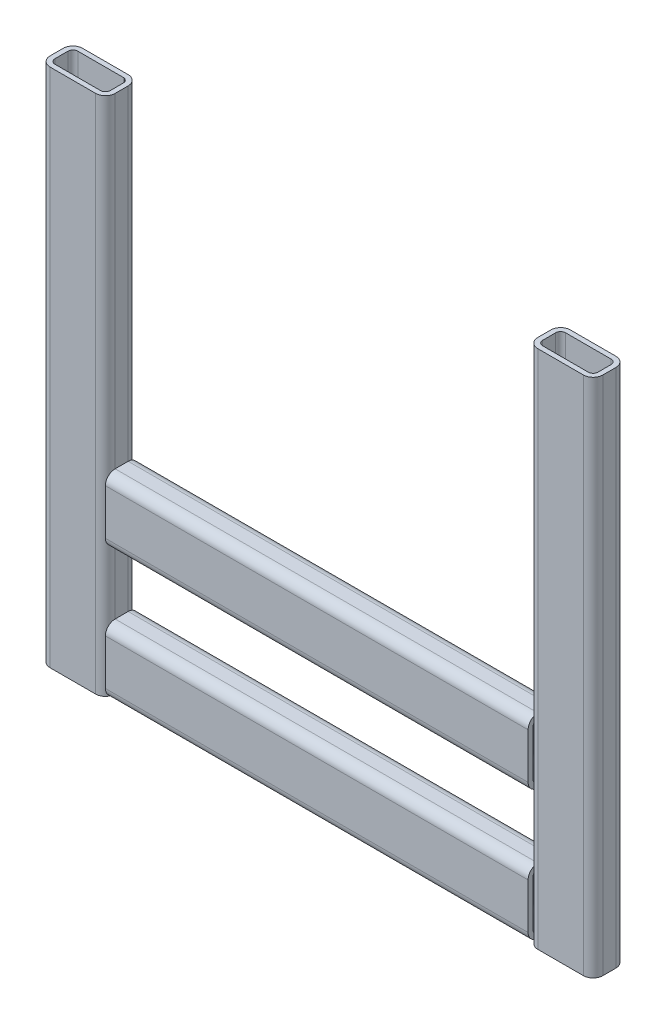
SolidWorks part; units mm, degrees
material "普通碳钢"
ref_plane "前视基准面" through (0, 0, 0) normal (0, 0, 1) x (1, 0, 0)
ref_plane "上视基准面" through (0, 0, 0) normal (0, 1, 0) x (1, 0, 0)
ref_plane "右视基准面" through (0, 0, 0) normal (1, 0, 0) x (0, 0, -1)
sketch3d "3D草图1"
  line L0 (0, 0, 0) -> (300, 0, 0)
  line L1 (300, 0, 0) -> (300, 300, 0)
  line L2 (0, 0, 0) -> (0, 300, 0)
  line L3 (0, 80, 0) -> (300, 80, 0)
  dimension "D1" = 300
  dimension "D2" = 300
  dimension "D3" = 80
other "矩形管 40 X 20 X 3(1)"
ref_plane "基准面1" through (0, 0, 0) normal (0, 1, 0) x (0, 0, -1)
sketch "Sketch1" plane through (0, 0, 0) normal (0, 1, 0) x (0, 0, -1)
  line L0 (-4, -17) -> (4, -17)
  line L1 (-7, -14) -> (-7, 14)
  line L2 (4, 17) -> (-4, 17)
  line L3 (7, 14) -> (7, -14)
  line L4 (-4, -20) -> (4, -20)
  line L5 (-10, -14) -> (-10, 14)
  line L6 (4, 20) -> (-4, 20)
  line L7 (10, 14) -> (10, -14)
  arc A0 (10, 14) -> (4, 20) centre (4, 14) ccw
  arc A1 (4, -20) -> (10, -14) centre (4, -14) ccw
  arc A2 (-10, -14) -> (-4, -20) centre (-4, -14) ccw
  arc A3 (-4, 20) -> (-10, 14) centre (-4, 14) ccw
  arc A4 (-4, 17) -> (-7, 14) centre (-4, 14) ccw
  arc A5 (7, 14) -> (4, 17) centre (4, 14) ccw
  arc A6 (4, -17) -> (7, -14) centre (4, -14) ccw
  arc A7 (-7, -14) -> (-4, -17) centre (-4, -14) ccw
  point P0 (0, 20)
  point P1 (10, 0)
  point P2 (0, -20)
  point P3 (-10, 0)
  point P4 (-10, 20)
  point P5 (10, 20)
  point P6 (10, -20)
  point P7 (-10, -20)
  point P8 (0, 0)
  point P33 (0, 0)
  dimension "D1" = 6
  dimension "Thickness" = 3
  dimension "V_leg" = 40
  dimension "H_leg" = 20
